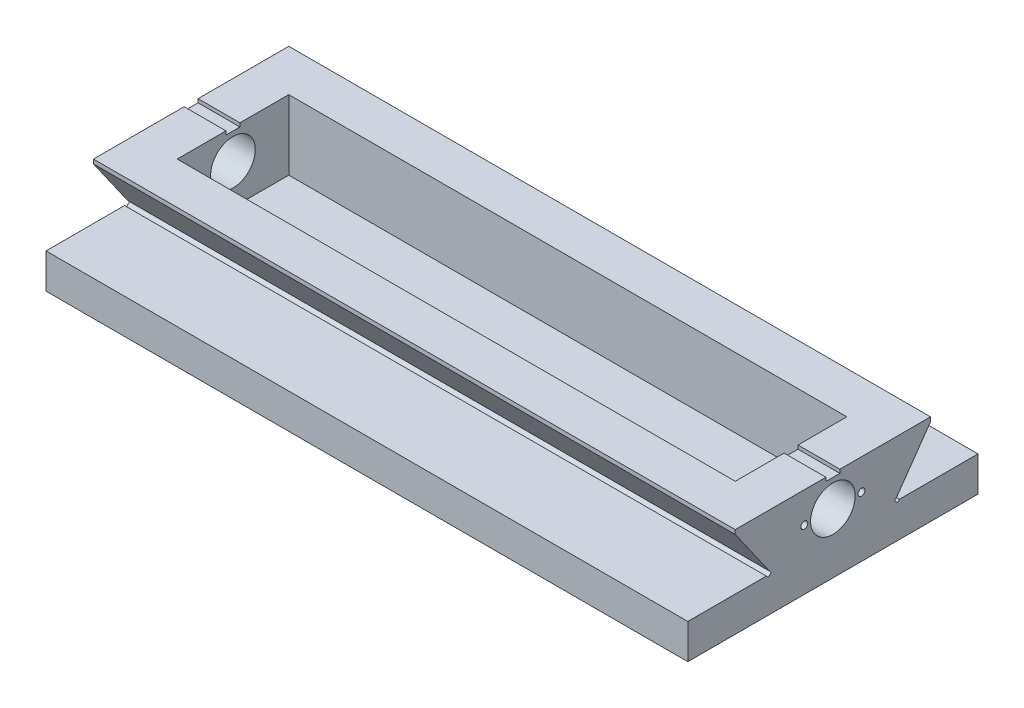
from build123d import *

# Parameters (mm, degrees)
BOSS_EXTRUDE1_DEPTH   = 460
SKETCH2_W             = 400
SKETCH2_H             = 80
CUT_EXTRUDE1_DEPTH    = 50
SKETCH3_R             = 16
CUT_EXTRUDE2_DEPTH    = 475.523181731
M6_TAPPED_HOLE1_D     = 5
M6_TAPPED_HOLE1_DEPTH = 17
M6_TAPPED_HOLE1_TIP   = 1.502151548
M6_TAPPED_HOLE2_D     = 5
M6_TAPPED_HOLE2_DEPTH = 17
M6_TAPPED_HOLE2_TIP   = 1.502151548


with BuildPart() as part:
    # Sketch1 → Boss-Extrude1 (new body)
    with BuildSketch(Plane(origin=(0, 0, 0), x_dir=(0, 0, -1), z_dir=(1, 0, 0))):
        Polygon((-104, 12.5), (-47.702939672, 12.5), (-46.297660938, 11.076907706), (-44.163022497, 13.184825808), (-45.568301231, 14.607918102), (-70, 49.5), (-70, 52.5), (-5, 52.5), (-5, 49.916740154), (5, 49.916740154), (5, 52.5), (70, 52.5), (70, 49.5), (45.568301231, 14.607918102), (44.163022497, 13.184825808), (46.297660938, 11.076907706), (47.702939672, 12.5), (104, 12.5), (104, -12.5), (-104, -12.5), align=None)
    extrude(amount=BOSS_EXTRUDE1_DEPTH)

    # Sketch2 → Cut-Extrude1 (cut)
    with BuildSketch(Plane(origin=(0, 52.5, 0), x_dir=(1, 0, 0), z_dir=(0, 1, 0))):
        with Locations((230, 0)):
            Rectangle(SKETCH2_W, SKETCH2_H)
    extrude(amount=-CUT_EXTRUDE1_DEPTH, mode=Mode.SUBTRACT)

    # Sketch3 → Cut-Extrude2 (cut, through all)
    with BuildSketch(Plane(origin=(460, 0, 0), x_dir=(0, 0, -1), z_dir=(1, 0, 0))):
        with Locations((0, 30.5)):
            Circle(SKETCH3_R)
    extrude(amount=-CUT_EXTRUDE2_DEPTH, mode=Mode.SUBTRACT)

    # M6 Tapped Hole1
    with Locations(Plane(origin=(460, 0, 0), x_dir=(0, 0, -1), z_dir=(1, 0, 0))):
        with Locations((-20.5, 30.5), (20.5, 30.5)):
            Hole(M6_TAPPED_HOLE1_D / 2, depth=M6_TAPPED_HOLE1_DEPTH)
            with Locations((0, 0, -(M6_TAPPED_HOLE1_DEPTH + M6_TAPPED_HOLE1_TIP / 2))):  # 118° drill point
                Cone(0, M6_TAPPED_HOLE1_D / 2, M6_TAPPED_HOLE1_TIP, mode=Mode.SUBTRACT)

    # M6 Tapped Hole2
    with Locations(Plane.ZY):
        with Locations((17.453686729, 19.747381031), (-17.453687008, 41.252618969)):
            Hole(M6_TAPPED_HOLE2_D / 2, depth=M6_TAPPED_HOLE2_DEPTH)
            with Locations((0, 0, -(M6_TAPPED_HOLE2_DEPTH + M6_TAPPED_HOLE2_TIP / 2))):  # 118° drill point
                Cone(0, M6_TAPPED_HOLE2_D / 2, M6_TAPPED_HOLE2_TIP, mode=Mode.SUBTRACT)


solid = part.part
